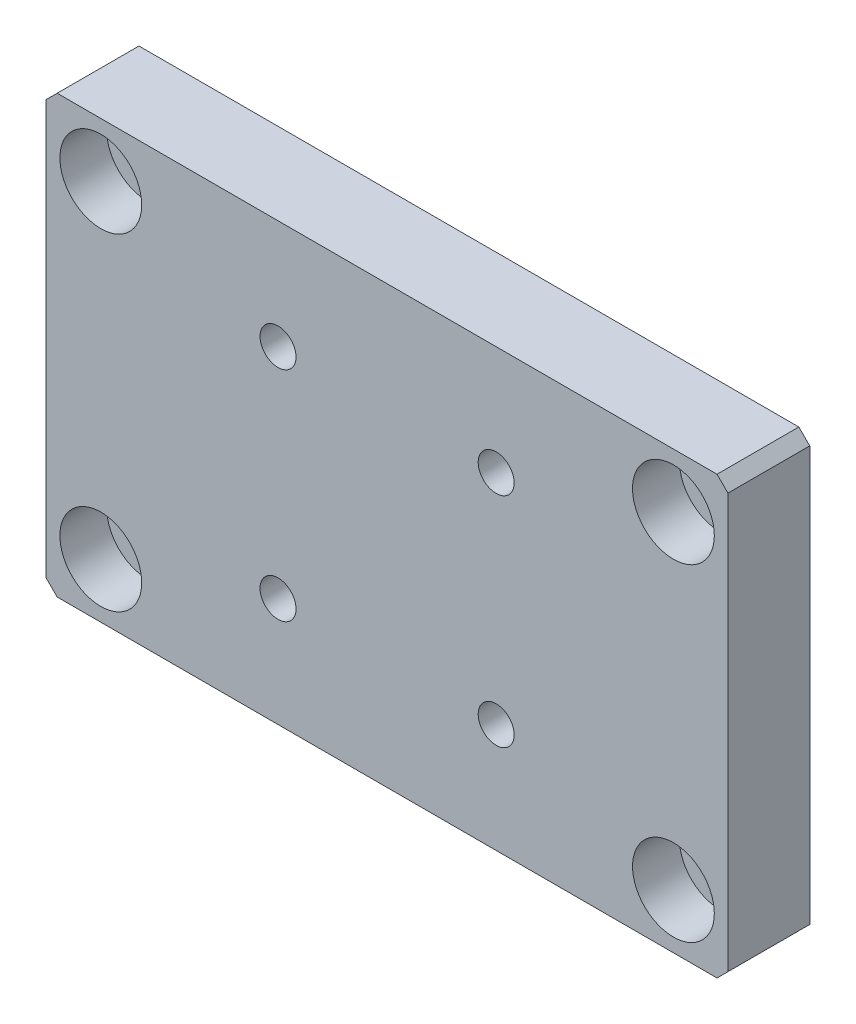
from build123d import *

# Parameters (mm, degrees)
SKETCH_1_W                   = 125
SKETCH_1_H                   = 80
EXTRUDE_1_DEPTH              = 7.5
HOLE_WIZARD_M8_1_D           = 9
HOLE_WIZARD_M8_1_CBORE_D     = 15
HOLE_WIZARD_M8_1_CBORE_DEPTH = 8.6
HOLE_WIZARD_M6_1_D           = 6.6
HOLE_WIZARD_M6_1_CBORE_D     = 11
HOLE_WIZARD_M6_1_CBORE_DEPTH = 6.4
CHAMFER_1_SIZE               = 2


with BuildPart() as part:
    # 草图1 → 凸台-拉伸1 (new, symmetric)
    with BuildSketch(Plane.XY):
        Rectangle(SKETCH_1_W, SKETCH_1_H)
    extrude(amount=EXTRUDE_1_DEPTH, both=True)

    # M8 六角凹头螺钉的柱形沉头孔1 (through all)
    with Locations(Plane.XY.offset(7.5)):
        with Locations((-52.5, 30), (-52.5, -30), (52.5, -30), (52.5, 30)):
            CounterBoreHole(HOLE_WIZARD_M8_1_D / 2, HOLE_WIZARD_M8_1_CBORE_D / 2, HOLE_WIZARD_M8_1_CBORE_DEPTH)

    # M6 六角凹头螺钉的柱形沉头孔1 (through all)
    with Locations(Plane(origin=(0, 0, -7.5), x_dir=(-1, 0, 0), z_dir=(0, 0, -1))):
        with Locations((-20, -20), (-20, 20), (20, -20), (20, 20)):
            CounterBoreHole(HOLE_WIZARD_M6_1_D / 2, HOLE_WIZARD_M6_1_CBORE_D / 2, HOLE_WIZARD_M6_1_CBORE_DEPTH)

    # 倒角1
    chamfer_1_edges = [part.edges().sort_by_distance(p)[0] for p in [
        (62.5, -40, 0),
        (-62.5, -40, 0),
        (-62.5, 40, 0),
        (62.5, 40, 0),
    ]]
    chamfer(chamfer_1_edges, length=CHAMFER_1_SIZE)


solid = part.part
